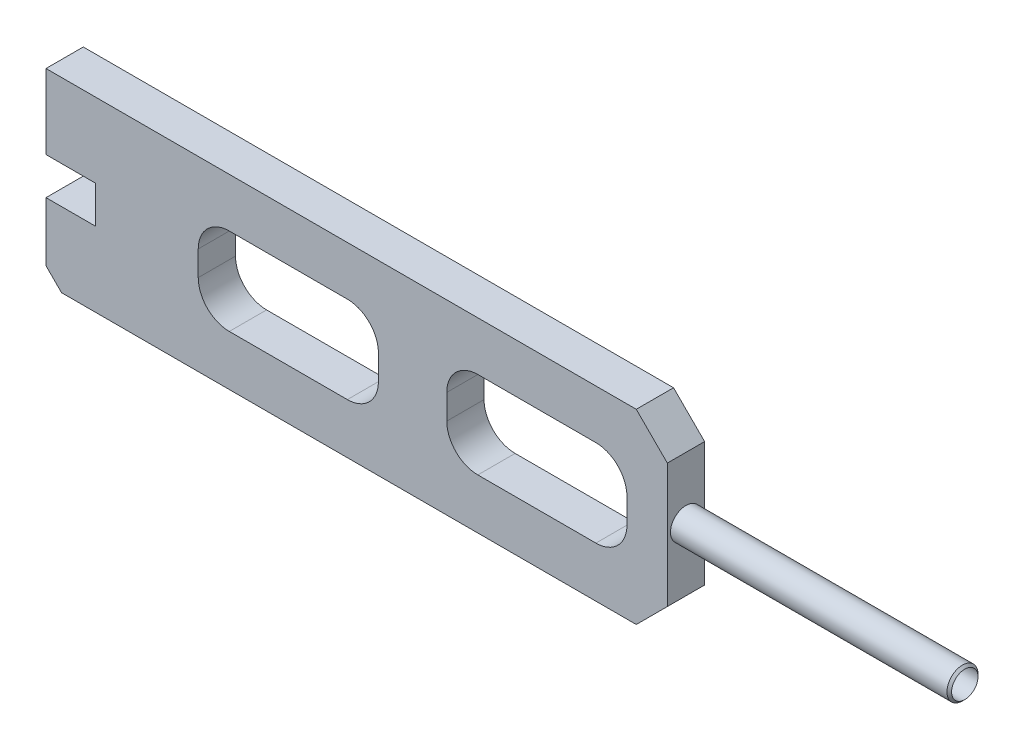
SolidWorks part; units mm, degrees
material "1023 碳钢板 (SS)"
ref_plane "Front Plane" through (0, 0, 0) normal (0, 0, 1) x (1, 0, 0)
ref_plane "Top Plane" through (0, 0, 0) normal (0, 1, 0) x (1, 0, 0)
ref_plane "Right Plane" through (0, 0, 0) normal (1, 0, 0) x (0, 0, -1)
ref_plane "Plane4" through (0, 0, 6) normal (0, 0, 1) x (1, 0, 0)
sketch "Sketch1" plane through (0, 0, 6) normal (0, 0, 1) x (1, 0, 0)
  line L0 (-100, 30) -> (-100, -30)
  line L1 (-100, -30) -> (100, -30)
  line L2 (100, -30) -> (100, 30)
  line L3 (100, 30) -> (-100, 30)
extrude "Boss-Extrude1" add sketch "Sketch1" against normal blind 12
sketch "Sketch2" plane through (0, 0, -6) normal (0, 0, -1) x (-1, 0, 0)
  line L0 (100, 6) -> (84, 6)
  line L1 (84, 6) -> (84, -6)
  line L2 (84, -6) -> (100, -6)
  line L3 (100, -6) -> (100, 6)
  point P4 (84, 0)
extrude "Cut-Extrude1" cut sketch "Sketch2" against normal through all
sketch "Sketch3" plane through (0, 0, 6) normal (0, 0, 1) x (1, 0, 0)
  line L0 (-51, -13.8) -> (7, -13.8)
  line L1 (7, -13.8) -> (7, 14.2)
  line L2 (7, 14.2) -> (-51, 14.2)
  line L3 (-51, 14.2) -> (-51, -13.8)
extrude "Cut-Extrude2" cut sketch "Sketch3" against normal through all
sketch "Sketch4" plane through (0, 0, -6) normal (0, 0, -1) x (-1, 0, 0)
  line L0 (-29, 14.2) -> (-87, 14.2)
  line L1 (-87, 14.2) -> (-87, -13.8)
  line L2 (-87, -13.8) -> (-29, -13.8)
  line L3 (-29, -13.8) -> (-29, 14.2)
extrude "Cut-Extrude3" cut sketch "Sketch4" against normal through all
ref_plane "Plane5" through (0, 0, 0) normal (0, 0, -1) x (-1, 0, 0)
sketch "Sketch5" plane through (0, 0, 0) normal (0, 0, -1) x (-1, 0, 0)
  line L0 (-190, 5.2) -> (-190, 0.2)
  line L1 (-190, 0.2) -> (-100, 0.2)
  line L2 (-100, 0.2) -> (-100, 5.2)
  line L3 (-100, 5.2) -> (-190, 5.2)
  line L4 (-190, 0.2) -> (-100, 0.2) construction
revolve "Revolve1" add sketch "Sketch5" angle 360 about L4
hole_wizard "M6 Tapped Hole1" positions "Sketch7" profile "Sketch6" tap size "M6" standard "GB"
sketch "Sketch7" plane through (-100, 0, 0) normal (-1, 0, 0) x (0, 0, 1)
  point P0 (0, 18)
cosmetic thread "Cosmetic Thread1" parameters "D1"=10, "D2"=6
sketch "Sketch6" plane through (-100, 18, 0) normal (0, 1, 0) x (0, 0, 1)
  line L0 (0, 0) -> (0, 14.5022)
  line L1 (0, 14.5022) -> (2.5, 13)
  line L2 (2.5, 13) -> (2.5, 0)
  line L5 (2.5, 0) -> (0, 0)
  line L10 (0, 14.5022) -> (-2.5, 13) construction
  line L11 (0, -6.35) -> (0, 107.95) construction
  dimension "螺纹孔钻头直径" = 5
  dimension "螺纹孔钻头深度" = 13
  dimension "导头角度" = 118
chamfer "Chamfer1" distance 1 angle 45 1 edges at (190, 0.2, 5)
chamfer "Chamfer2" distance 10 angle 45 2 edges at (100, 30, 0) (100, -30, 0)
chamfer "Chamfer3" distance 5 angle 45 1 edges at (-100, -30, 0)
fillet "Fillet1" radius 10 8 edges at (-51, -13.8, 0) (7, 14.2, 0) (-51, 14.2, 0) (29, -13.8, 0) (7, -13.8, 0) (87, 14.2, 0) (87, -13.8, 0) (29, 14.2, 0)
sketch "Sketch10" plane through (190, 0, 0) normal (1, 0, 0) x (0, 0, -1)
  circle A0 centre (0, 0.2) radius 2.296
hole_wizard "M10 Tapped Hole1" positions "Sketch15" profile "Sketch16" tap size "M10" standard "GB"
sketch "Sketch15" plane through (190, 0, 0) normal (1, 0, 0) x (0, 0, -1)
  point P0 (0, 0.2)
cosmetic thread "Cosmetic Thread2" parameters "D1"=95, "D2"=10
sketch "Sketch16" plane through (190, 0.2, 0) normal (0, 1, 0) x (0, 0, -1)
  line L0 (0, 0) -> (0, 102.0537)
  line L1 (0, 102.0537) -> (4.25, 99.5)
  line L2 (4.25, 99.5) -> (4.25, 0)
  line L5 (4.25, 0) -> (0, 0)
  line L10 (0, 102.0537) -> (-4.25, 99.5) construction
  line L11 (0, -6.35) -> (0, 107.95) construction
  dimension "螺纹孔钻头直径" = 8.5
  dimension "螺纹孔钻头深度" = 99.5
  dimension "导头角度" = 118
ref_plane "Plane6" through (-92, 0, 0) normal (-1, 0, 0) x (0, 0, 1)
